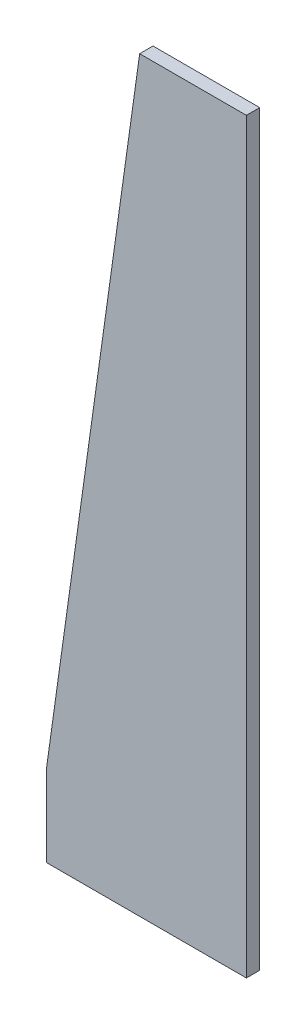
from build123d import *

# Parameters (mm, degrees)
EXTRUDE_3_DEPTH = 5


with BuildPart() as part:
    # 草图1 → 凸台-拉伸3 (new body)
    with BuildSketch(Plane.XY):
        Polygon((-5, 0), (0, 0), (70, 0), (70, 280), (30, 280), (-5, 30), align=None)
    extrude(amount=EXTRUDE_3_DEPTH)


solid = part.part
